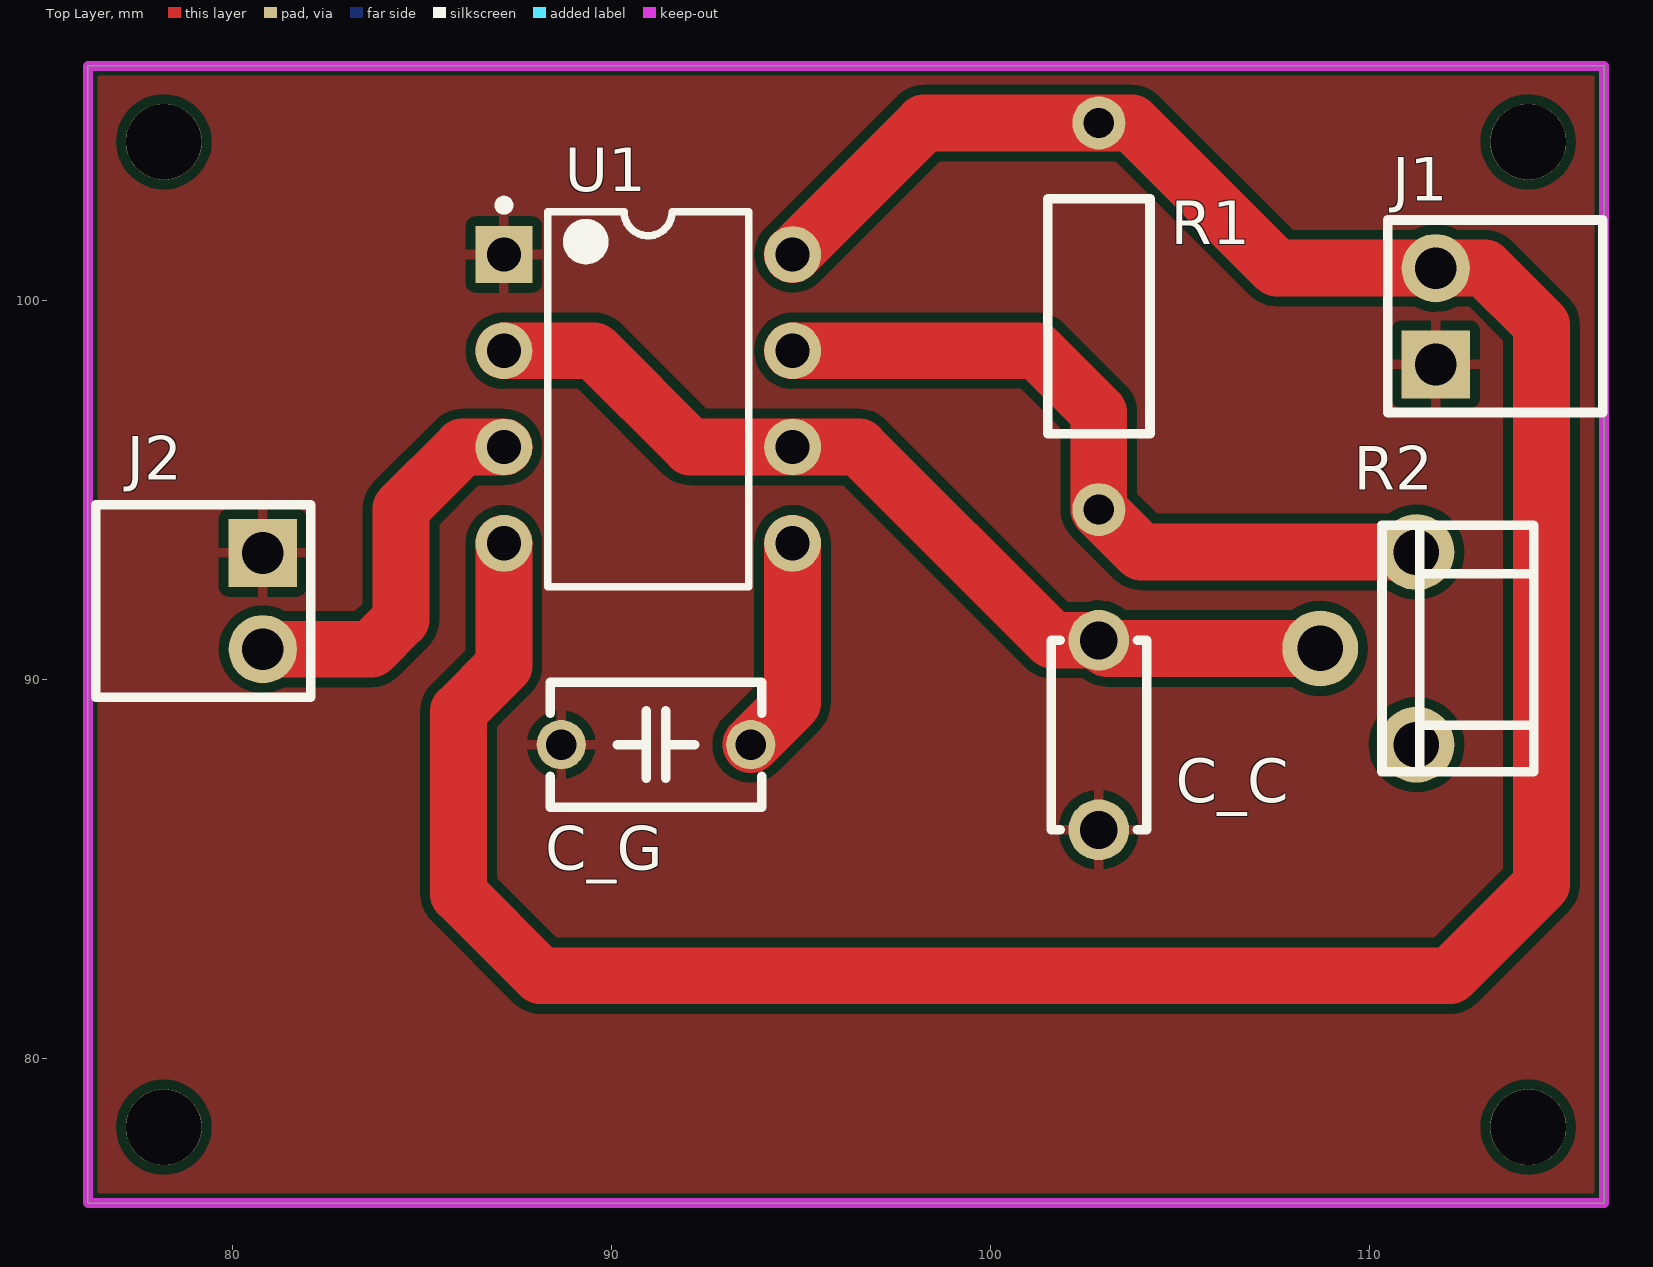
[diagram p0: Top Layer view]
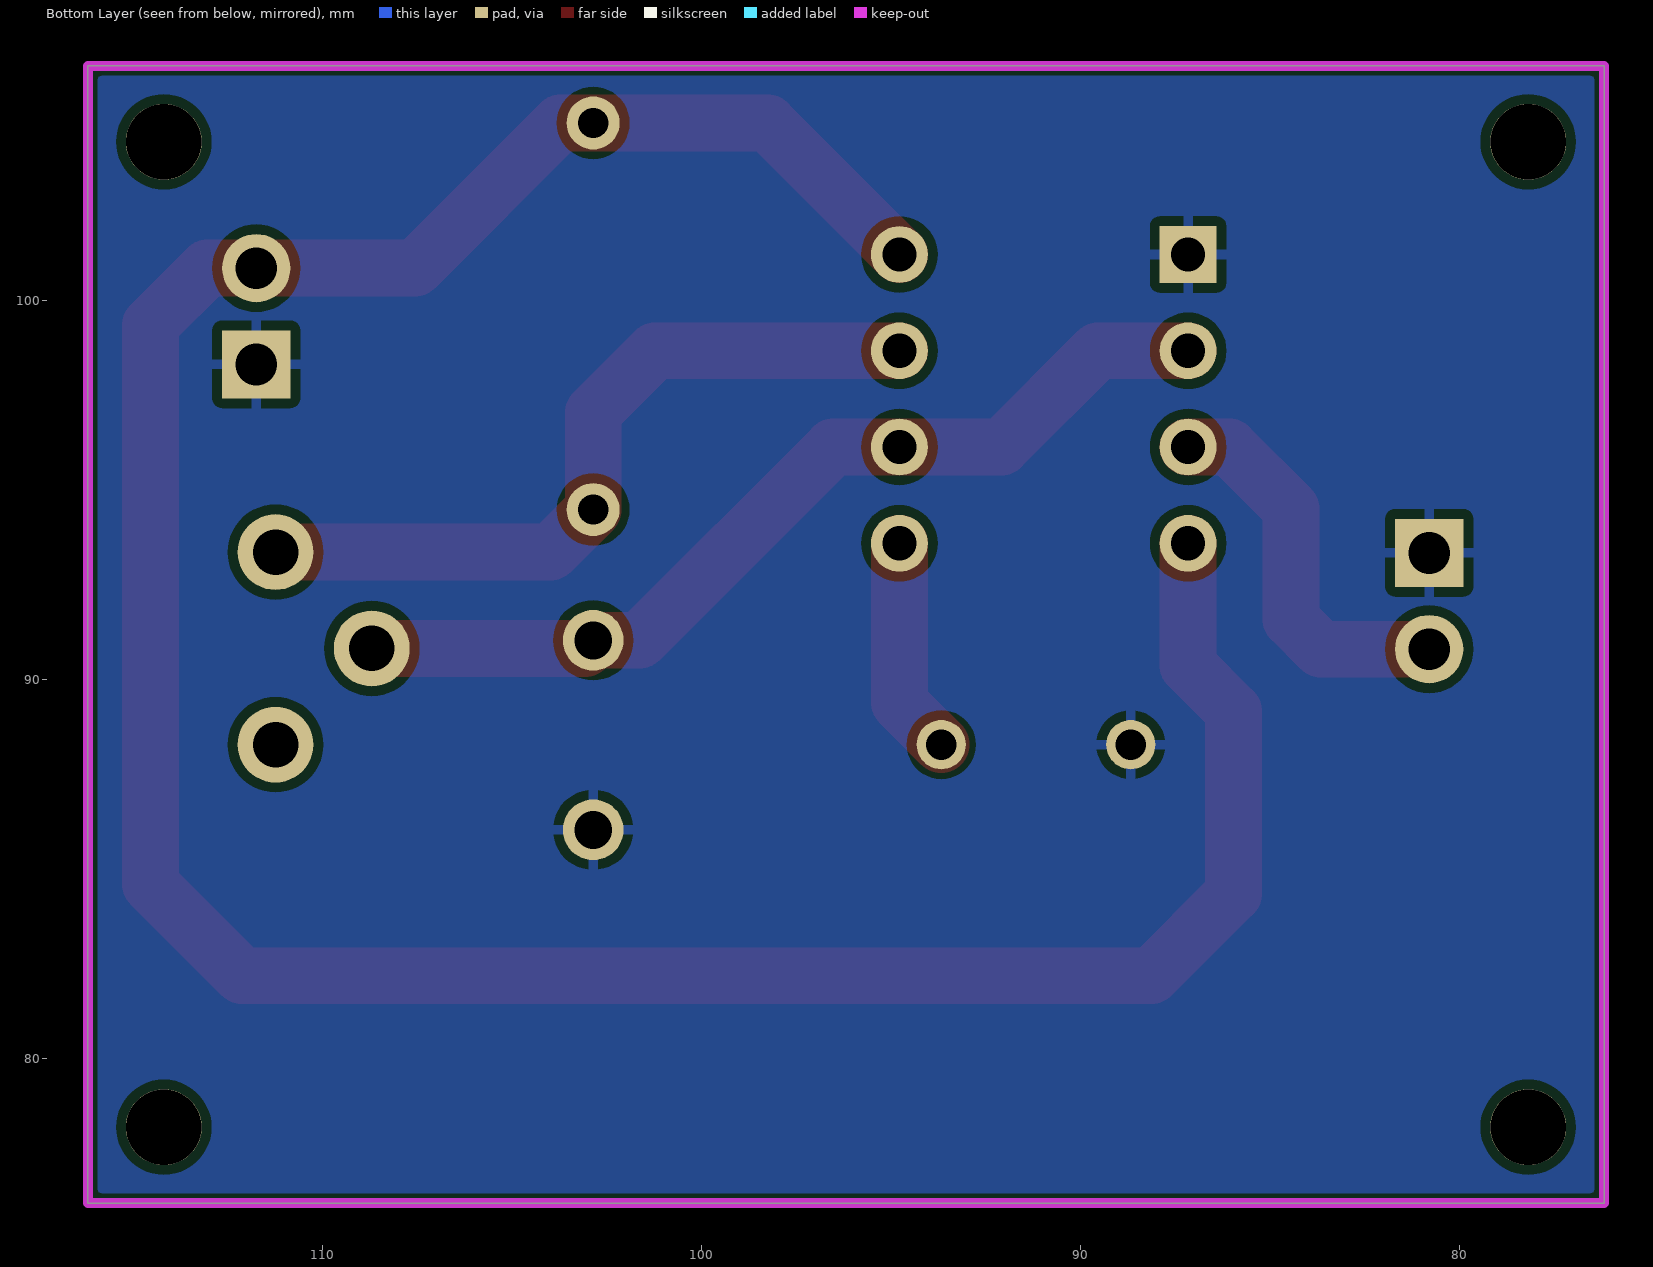
[diagram p1: Bottom Layer view, seen from below]
# Altium PCB MISC51049.pcbdoc
Units mm, origin at the board's own origin, x right, y up, seen from the top; angles counter-clockwise.
Board outline 40 x 30 mm, 2 copper layers (Top Layer, Bottom Layer), stack 1.58 mm thick; 7 components, 6 nets, 25 pads, 0 vias.

## Layer stack, top to bottom
Top Solder Mask Layer: solder mask 0.01, Dk 3.3
Top Layer: signal copper 0.035
Dielectric1: surface 1.51, FR4, Dk 4.5
Bottom Layer: signal copper 0.035
Bottom Solder Mask Layer: solder mask 0.01, Dk 3.3

## Board outline
76.2,106.2 76.2,76.2 116.2,76.2 116.2,106.2

## Design rules (kind name [scope] priority, off if disabled: settings)
BoardOutlineClearance copperThickness2oz_1 [All] p2 off: genericclearance=0.203 ignorepadtopadclearanceinfootprint=FALSE except(0: Arc-SplitContinuation Track-SplitContinuation SMDPad-SplitContinuation THPad-SplitContinuation Via-SplitContinuation Fill-SplitContinuation Region-SplitContinuation Poly-SplitContinuation Text-SplitContinuation Hole-SplitContinuation; 0.152: Arc-CutoutEdge SMDPad-CutoutEdge THPad-CutoutEdge Via-CutoutEdge Fill-CutoutEdge Region-CutoutEdge Text-CutoutEdge; 0.176: Hole-OutlineEdge Hole-CutoutEdge; 0.254: Poly-OutlineEdge Poly-CutoutEdge; 0.3: Arc-OutlineEdge Track-OutlineEdge SMDPad-OutlineEdge THPad-OutlineEdge Via-OutlineEdge Fill-OutlineEdge Region-OutlineEdge Text-OutlineEdge Track-CutoutEdge)
BoardOutlineClearance copperThickness1oz_1 [All] p4: genericclearance=0.102 ignorepadtopadclearanceinfootprint=FALSE except(0: Arc-SplitContinuation Track-SplitContinuation SMDPad-SplitContinuation THPad-SplitContinuation Via-SplitContinuation Fill-SplitContinuation Region-SplitContinuation Poly-SplitContinuation Text-SplitContinuation Hole-SplitContinuation; 0.152: SMDPad-CutoutEdge THPad-CutoutEdge Via-CutoutEdge Fill-CutoutEdge Region-CutoutEdge Text-CutoutEdge; 0.176: Hole-OutlineEdge Hole-CutoutEdge; 0.254: Poly-OutlineEdge Poly-CutoutEdge; 0.3: Arc-OutlineEdge Track-OutlineEdge SMDPad-OutlineEdge THPad-OutlineEdge Via-OutlineEdge Fill-OutlineEdge Region-OutlineEdge Text-OutlineEdge Arc-CutoutEdge Track-CutoutEdge)
Clearance copperThickness2oz [All] p1 off: gap=0.203 ignorepadtopadclearanceinfootprint=FALSE except(0.152: SMDPad-Track SMDPad-SMDPad THPad-Track SMDPad-THPad THPad-THPad Track-Via SMDPad-Via THPad-Via Via-Via Fill-Track Region-Track Fill-SMDPad Region-SMDPad Fill-THPad Region-THPad Fill-Via Region-Via Fill-Fill Fill-Region Region-Region Arc-Track Arc-SMDPad Arc-THPad Arc-Via Fill-Arc Region-Arc Arc-Arc Text-Track SMDPad-Text Text-THPad Text-Via Fill-Text Region-Text Arc-Text Text-Text; 0.176: Hole-Track Hole-SMDPad Hole-THPad Hole-Via Fill-Hole Region-Hole Hole-Arc Hole-Text; 0.254: Poly-Track Poly-SMDPad Poly-THPad Poly-Via Poly-Fill Poly-Region Poly-Poly Poly-Arc Poly-Text Poly-Hole)
Clearance copperThickness1oz [All] p3: gap=0.102 ignorepadtopadclearanceinfootprint=FALSE except(0.152: SMDPad-Track SMDPad-SMDPad THPad-Track SMDPad-THPad THPad-THPad Track-Via SMDPad-Via THPad-Via Via-Via Fill-Track Region-Track Fill-SMDPad Region-SMDPad Fill-THPad Region-THPad Fill-Via Region-Via Fill-Fill Fill-Region Region-Region Arc-Track Arc-SMDPad Arc-THPad Arc-Via Fill-Arc Region-Arc Arc-Arc Text-Track SMDPad-Text Text-THPad Text-Via Fill-Text Region-Text Arc-Text Text-Text; 0.176: Hole-Track Hole-SMDPad Hole-THPad Hole-Via Fill-Hole Region-Hole Hole-Arc Hole-Text; 0.254: Poly-Track Poly-SMDPad Poly-THPad Poly-Via Poly-Fill Poly-Region Poly-Poly Poly-Arc Poly-Text Poly-Hole)
Creepage creepage [All] p1: checkdistance=0 ignoreinternallayers=TRUE applytopolygonpour=TRUE
DiffPairsRouting differentialPair [All] p1: maxlimit=0.152 minlimit=0.152 mostfreqgap=0.152 toplayer_minwidth=0.127 toplayer_prefwidth=0.254 toplayer_maxwidth=2.54 toplayer_mingap=0.152 toplayer_prefgap=0.152 toplayer_maxgap=0.152 bottomlayer_minwidth=0.127 bottomlayer_prefwidth=0.254 bottomlayer_maxwidth=2.54 bottomlayer_mingap=0.152 bottomlayer_prefgap=0.152 bottomlayer_maxgap=0.152 maxuncoupledlength=0.254
HoleToHoleClearance otherClearance [All] p1: gap=0.3 allowstackedmicrovias=TRUE
Length netLength [All] p1: minlimit=0 maxlimit=0
MatchedLengths netLengthTolerance [All] p1: tolerance=25.4
PasteMaskExpansion pasteMaskExpansion [All] p1: expansion=0
PlaneConnect innerPlane [All] p1: planeconnectstyle=Relief reliefexpansion=0.508 reliefentries=4 reliefconductorwidth=0.254 reliefairgap=0.254
PolygonConnect copperRegion [(InNet('GND'))] p1: connectstyle=Relief reliefconductorwidth=0.254 reliefentries=4 polygonreliefangle="90 Angle" airgapwidth=0.254 via.connectstyle=Relief via.reliefconductorwidth=0.254 via.reliefentries=4 via.polygonreliefangle="90 Angle" via.airgapwidth=0.254
RoutingVias viaSize [All] p1: holewidth=0.305 width=0.61 viastyle="Through Hole" minholewidth=0.3 minwidth=0.5 maxholewidth=6.3 maxwidth=10
SolderMaskExpansion solderMaskExpansion [IsVia] p1: expansion=-25.4 istentingtop=TRUE
SolderMaskExpansion solderMaskExpansion [All] p2: expansion=0.051 istentingtop=FALSE
Width copperThickness2oz_2 [All] p1 off: maxlimit=2.54 minlimit=0.203 preferedwidth=0.254
Width copperThickness1oz_2 [All] p2: maxlimit=2.54 minlimit=0.127 preferedwidth=0.254

## Components (designator, comment, footprint, x,y, rotation, side; value= is the part's Value field where it differs from the comment)
C_C "100nF" CAP-TH_L5.0-W2.5-P5.00-D1.0 102.87,88.547 r90 top
C_G "10nF" CAP-TH_L5.5-W3.0-P5.00-D0.6 91.186,88.293 r0 top
J1 "" HDR-TH_2P-P2.54-V-M-1 111.76,99.596 r90 top
J2 "" HDR-TH_2P-P2.54-V-M-1 80.812,92.082 r270 top
R1 "1kΩ" RES-TH_BD2.7-L6.2-P10.20-D0.4 102.87,99.596 r90 top
R2 "1MΩ" RES-ADJ-TH_RM063-103 109.982,90.833 r90 top
U1 "NE555P" DIP-8_L9.8-W6.6-P2.54-LS7.6-BL 90.982,97.416 r270 top

## Footprints (in the part's own frame and the unit in brackets; to place one, negate y for a bottom-side part, rotate by r counter-clockwise, add the part's x,y. Pads: shape width x height; smd on the part's side, far side on the other; paste and mask are expansions set on the pad)
CAP-TH_L5.0-W2.5-P5.00-D1.0 [mm]
  round 1.6 hole 1: 1(-2.5,0) 2(2.5,0)
  silkscreen extent -2.5,-1.27 2.5,1.25
CAP-TH_L5.5-W3.0-P5.00-D0.6 [mm]
  round 1.3 hole 0.8 paste+0 mask+0.05: 1(-2.5,0) 2(2.5,0)
  silkscreen extent -2.79,-1.65 2.79,1.65
DIP-8_L9.8-W6.6-P2.54-LS7.6-BL [mm]
  rect 1.5x1.5 hole 0.9: 1(-3.81,-3.81)
  round 1.5 hole 0.9: 2(-1.27,-3.81) 3(1.27,-3.81) 4(3.81,-3.81) 5(3.81,3.81) 6(1.27,3.81) 7(-1.27,3.81) 8(-3.81,3.81)
  silkscreen extent -5.23,-3.93 4.96,2.65
HDR-TH_2P-P2.54-V-M-1 [mm]
  rect 1.8x1.8 hole 1.1: 1(-1.27,0)
  round 1.8 hole 1.1: 2(1.27,0)
  silkscreen extent -2.54,-4.41 2.54,1.27
RES-ADJ-TH_RM063-103 [mm]
  round 2 hole 1.2 paste+0 mask+0.05: 1(-2.54,-1.27) 2(0,1.27) 3(2.54,-1.27)
  silkscreen extent -3.25,-4.36 3.25,-0.36
RES-TH_BD2.7-L6.2-P10.20-D0.4 [mm]
  round 1.4 hole 0.8 copper offset 0,0: 1(-5.1,0) 2(5.1,0)
  silkscreen extent -3.1,-1.35 3.1,1.35

## Free pads (board coordinates)
  round 2 hole 2: 1(78.2,78.2) 1(78.2,104.2) 1(114.2,78.2) 1(114.2,104.2)

## Nets (pads, with @x,y where several pads share a name; then routed paths per layer and width w, separated by ;. In a path a pad name is that pad's centre, name@x,y a point inside that pad or via, vN(x,y) a via of type N, cw(c..) or ccw(c..) an arc to the next point about the centre after c; other vN are vias at no path point)
$1N14: C_G.2 U1.5 | length 5.8
  Top Layer w1.5: C_G.2 94.792,89.399 U1.5
$1N15: C_C.2 R2.2 U1.2 U1.6 | length 24.8
  Top Layer w1.5: U1.2 89.556,98.686 92.096,96.146 U1.6 96.541,96.146 101.64,91.047 C_C.2 103.084,90.833 R2.2
$1N16: R1.1 R2.3 U1.7 | length 20.2
  Top Layer w1.5: U1.7 101.24,98.686 102.87,97.056 R1.1 103.993,93.373 R2.3
$1N20: J2.2 U1.3 | length 10.3
  Top Layer w1.5: J2.2 83.672,90.812 84.455,91.595 84.455,94.516 86.085,96.146 U1.3
GND: C_C.1 C_G.1 J1.1 J2.1 U1.1
VCC: J1.2 R1.2 U1.4 U1.8 | length 78.4
  Top Layer w1.5: U1.4 87.172,90.375 85.979,89.182 85.979,84.356 88.138,82.197 112.141,82.197 114.554,84.61 114.554,99.366 113.054,100.866 J1.2 107.569,100.866 103.739,104.696 R1.2 98.262,104.696 U1.8
pads on no net: R2.1

## Polygon pours and split planes (outlines as drawn)
GND on Top Layer (solid, remove dead copper, pour order 0): 76.2,106.2 76.2,76.2 116.2,76.2 116.2,106.2
GND on Bottom Layer (solid, remove dead copper, pour order 2): 76.2,106.2 76.2,76.2 116.2,76.2 116.2,106.2

## Keep-outs
Board Outline Layer:
  the board outline again, w0.254